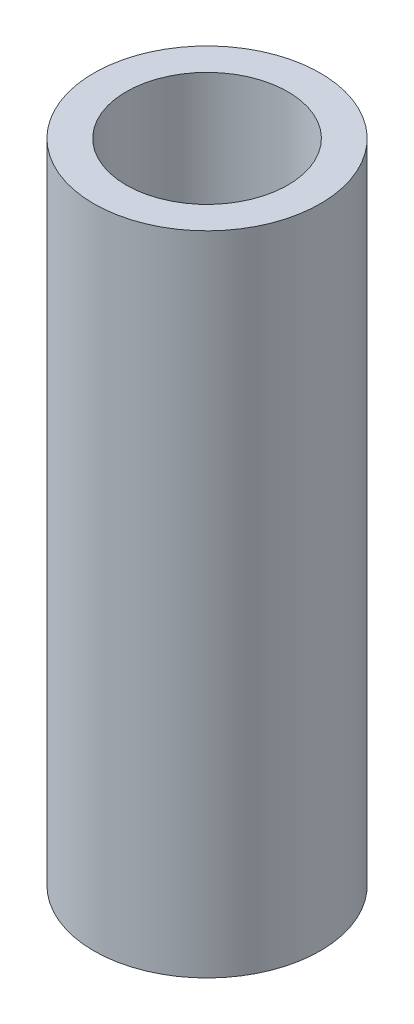
SolidWorks part; units mm, degrees
material "20#"
ref_plane "Front Plane" through (0, 0, 0) normal (0, 0, 1) x (1, 0, 0)
ref_plane "Top Plane" through (0, 0, 0) normal (0, 1, 0) x (1, 0, 0)
ref_plane "Right Plane" through (0, 0, 0) normal (1, 0, 0) x (0, 0, -1)
sketch "Sketch1" plane through (0, 0, 0) normal (0, 1, 0) x (1, 0, 0)
  circle A0 centre (0, 0) radius 17.5
  circle A1 centre (0, 0) radius 12.5
  dimension "D1" = 35
  dimension "D2" = 25
extrude "Boss-Extrude1" add sketch "Sketch1" along normal blind 100
fillet "Fillet1" radius 2 1 edges at (0, 0, 12.5)
